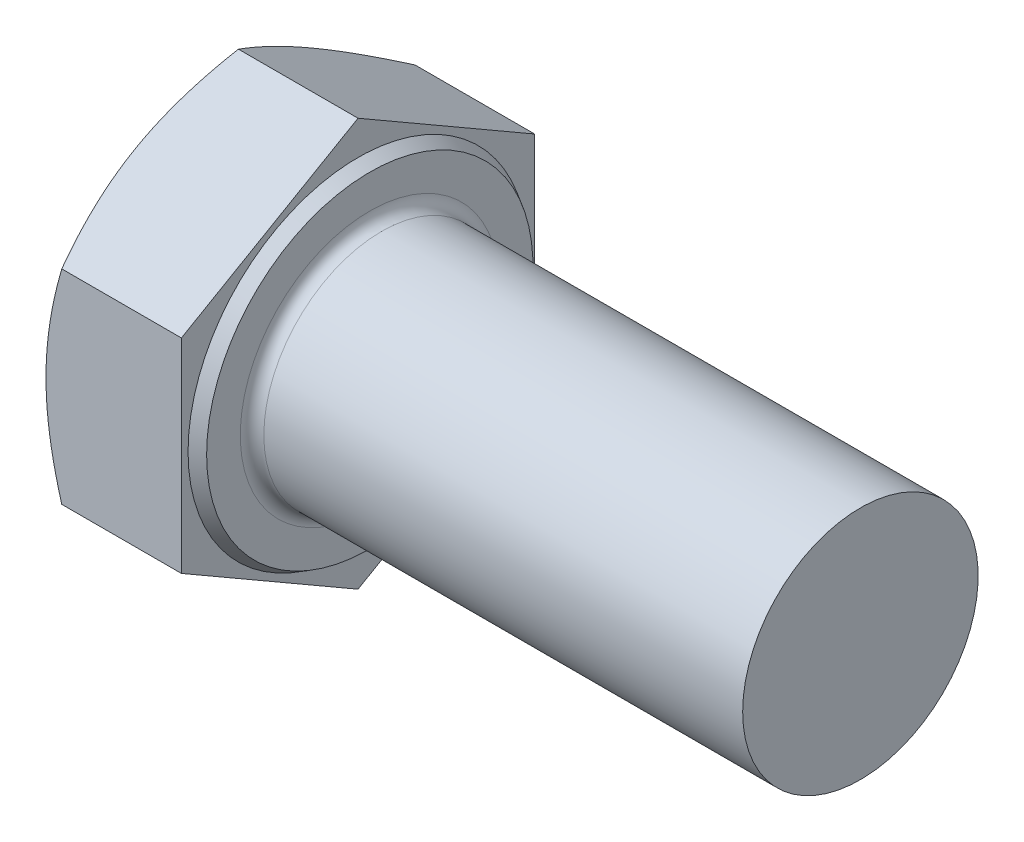
from build123d import *

# Parameters (mm, degrees)
EXTRUDE_387_DEPTH = 7.5
FILLET_1280_R     = 0.6


with BuildPart() as part:
    # 草图1 → Extrude 387 (new body)
    with BuildSketch(Plane(origin=(0, 0, 0), x_dir=(0, 0, -1), z_dir=(1, 0, 0))):
        Polygon((9, 5.196152423), (9, -5.196152423), (0, -10.392304845), (-9, -5.196152423), (-9, 5.196152423), (0, 10.392304845), align=None)
    extrude(amount=EXTRUDE_387_DEPTH)

    # 草图2 → 凸台-旋转1 (revolve)
    with BuildSketch(Plane.XY, mode=Mode.PRIVATE) as revolve_1_sk:
        Polygon((0, 0), (32.5, 0), (32.5, 4.4845), (32.5, 6), (2.5, 6), (0, 6), align=None)
    revolve(revolve_1_sk.sketch.rotate(Axis((0, 0, 0), (1, 0, 0)), 90), axis=Axis((0, 0, 0), (1, 0, 0)))

    # 草图3 → 切除-旋转1 (revolve, cut)
    with BuildSketch(Plane.XY):
        Polygon((0, 9), (3.690598923, 15.392304845), (3.690598923, 20.392304845), (-10, 20.392304845), (-10, 9), align=None)
    revolve(axis=Axis((0, 0, 0), (1, 0, 0)), mode=Mode.SUBTRACT)

    # 草图4 → 切除-旋转3 (revolve, cut)
    with BuildSketch(Plane.XY, mode=Mode.PRIVATE) as cut_revolve_3_sk:
        Polygon((7.5, 8.315), (6.9, 8.661410162), (6.9, 10.392304845), (7.5, 10.392304845), align=None)
    revolve(cut_revolve_3_sk.sketch.rotate(Axis((0, 0, 0), (1, 0, 0)), 90), axis=Axis((0, 0, 0), (1, 0, 0)), mode=Mode.SUBTRACT)

    # Fillet 1280
    fillet_1280_edges = [part.edges().sort_by_distance(p)[0] for p in [
        (7.5, 0, -6),
    ]]
    fillet(fillet_1280_edges, radius=FILLET_1280_R)


solid = part.part
